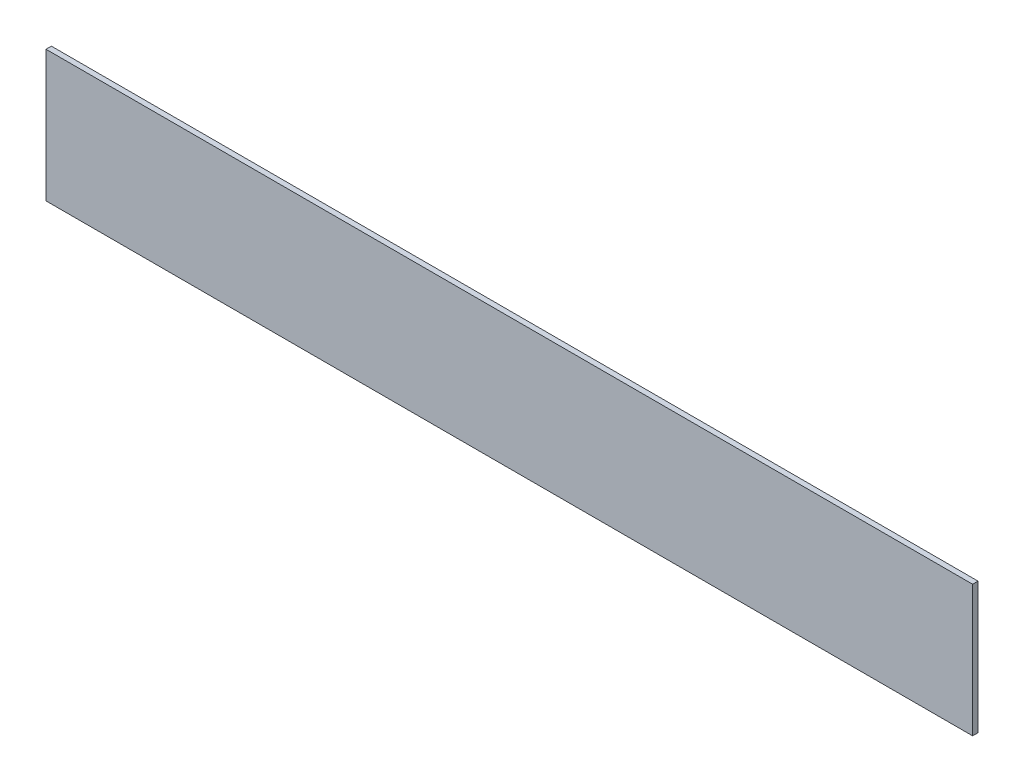
from build123d import *

# Parameters (mm, degrees)
SKETCH1_W           = 515
SKETCH1_H           = 73
BOSS_EXTRUDE1_DEPTH = 3


with BuildPart() as part:
    # Sketch1 → Boss-Extrude1 (new body)
    with BuildSketch(Plane.XY):
        Rectangle(SKETCH1_W, SKETCH1_H)
    extrude(amount=BOSS_EXTRUDE1_DEPTH)


solid = part.part
